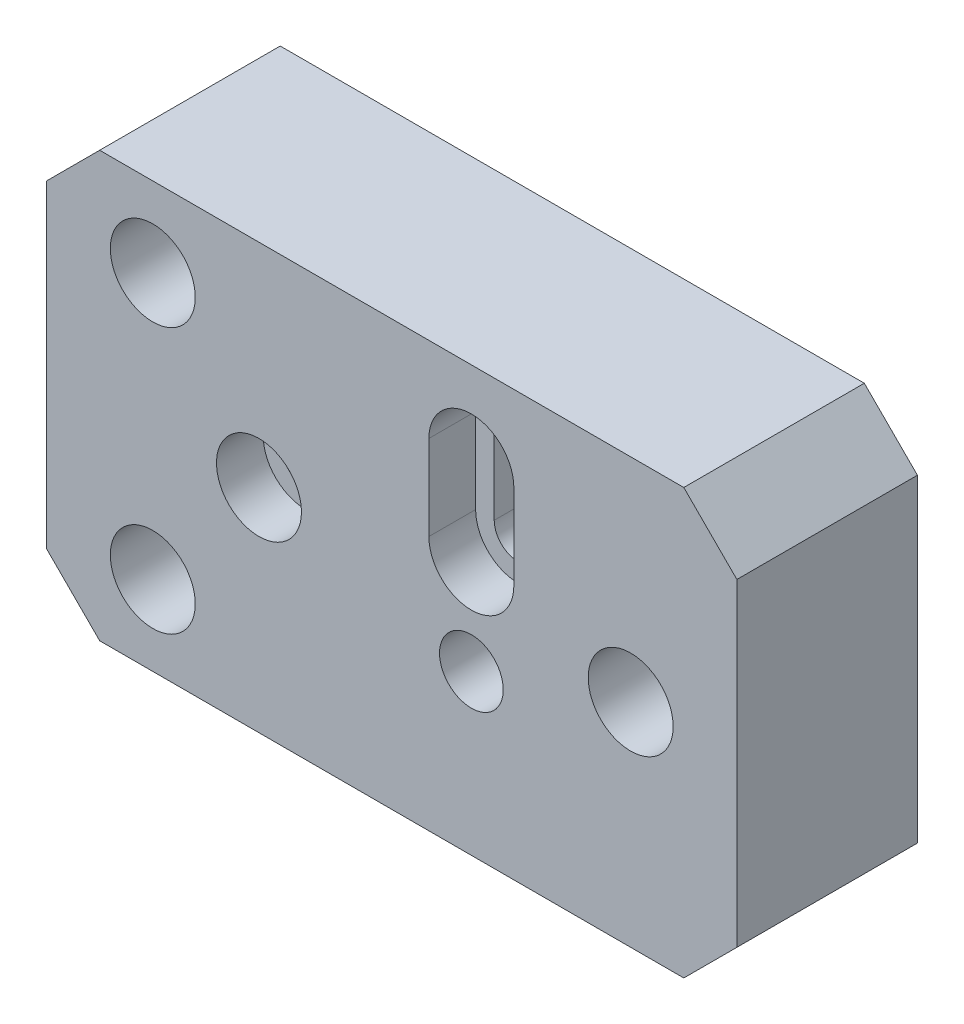
from build123d import *

# Parameters (mm, degrees)
SKETCH_1_W                   = 65
SKETCH_1_H                   = 40
EXTRUDE_1_DEPTH              = 8.5
HOLE_WIZARD_8_0_8_1_D        = 8
SKETCH_4_R                   = 6
CUT_EXTRUDE_1_DEPTH          = 9.5
HOLE_WIZARD_M4_1_D           = 4.5
HOLE_WIZARD_M4_1_CBORE_D     = 8
HOLE_WIZARD_M4_1_CBORE_DEPTH = 4.4
HOLE_WIZARD_6_0_6_1_D        = 6
CUT_EXTRUDE_2_DEPTH          = 9.5
CUT_EXTRUDE_3_DEPTH          = 42.776189391
CUT_EXTRUDE_START            = -4.4
CUT_EXTRUDE_4_DEPTH          = 4.4
CHAMFER_1_SIZE               = 5


with BuildPart() as part:
    # 草图1 → 凸台-拉伸1 (new, symmetric)
    with BuildSketch(Plane.XY):
        Rectangle(SKETCH_1_W, SKETCH_1_H)
    extrude(amount=EXTRUDE_1_DEPTH, both=True)

    # Ø8.0 (8) 直径孔1 (through all)
    with Locations(Plane.XY.offset(8.5)):
        with Locations((-22.5, 12.5), (-22.5, -12.5), (22.5, 0)):
            Hole(HOLE_WIZARD_8_0_8_1_D / 2)

    # 草图4 → 切除-拉伸1 (cut)
    with BuildSketch(Plane(origin=(0, 0, -8.5), x_dir=(-1, 0, 0), z_dir=(0, 0, -1))):
        with Locations((12.5, 0)):
            Circle(SKETCH_4_R)
    extrude(amount=-CUT_EXTRUDE_1_DEPTH, mode=Mode.SUBTRACT)

    # M4 六角凹头螺钉的柱形沉头孔1 (through all)
    with Locations(Plane.XY.offset(8.5)):
        with Locations((-12.5, 0)):
            CounterBoreHole(HOLE_WIZARD_M4_1_D / 2, HOLE_WIZARD_M4_1_CBORE_D / 2, HOLE_WIZARD_M4_1_CBORE_DEPTH)

    # Ø6.0 (6) 直径孔1 (through all)
    with Locations(Plane(origin=(0, 0, -8.5), x_dir=(-1, 0, 0), z_dir=(0, 0, -1))):
        with Locations((-7.5, -5)):
            Hole(HOLE_WIZARD_6_0_6_1_D / 2)

    # 草图9 → 切除-拉伸2 (cut)
    with BuildSketch(Plane(origin=(0, 0, -8.5), x_dir=(-1, 0, 0), z_dir=(0, 0, -1))):
        with BuildLine():
            Line((-11.5, 4), (-11.5, 12))
            ThreePointArc((-11.5, 12), (-7.5, 16), (-3.5, 12))
            Line((-3.5, 12), (-3.5, 4))
            ThreePointArc((-3.5, 4), (-7.5, 0), (-11.5, 4))
        make_face()
    extrude(amount=-CUT_EXTRUDE_2_DEPTH, mode=Mode.SUBTRACT)

    # 草图10 → 切除-拉伸3 (cut, through all)
    with BuildSketch(Plane.XY.offset(8.5)):
        with BuildLine():
            Line((5.25, 4), (5.25, 12))
            ThreePointArc((5.25, 12), (7.5, 14.25), (9.75, 12))
            Line((9.75, 12), (9.75, 4))
            ThreePointArc((9.75, 4), (7.5, 1.75), (5.25, 4))
        make_face()
    extrude(amount=-CUT_EXTRUDE_3_DEPTH, mode=Mode.SUBTRACT)

    # 草图11 → 切除-拉伸4 (cut)
    with BuildSketch(Plane.XY.offset(8.5).offset(CUT_EXTRUDE_START)):
        with BuildLine():
            Line((3.5, 4), (3.5, 12))
            ThreePointArc((3.5, 12), (7.5, 16), (11.5, 12))
            Line((11.5, 12), (11.5, 4))
            ThreePointArc((11.5, 4), (7.5, 0), (3.5, 4))
        make_face()
    extrude(amount=CUT_EXTRUDE_4_DEPTH, mode=Mode.SUBTRACT)

    # 倒角1
    chamfer_1_edges = [part.edges().sort_by_distance(p)[0] for p in [
        (32.5, -20, 0),
        (-32.5, -20, 0),
        (-32.5, 20, 0),
        (32.5, 20, 0),
    ]]
    chamfer(chamfer_1_edges, length=CHAMFER_1_SIZE)


solid = part.part
